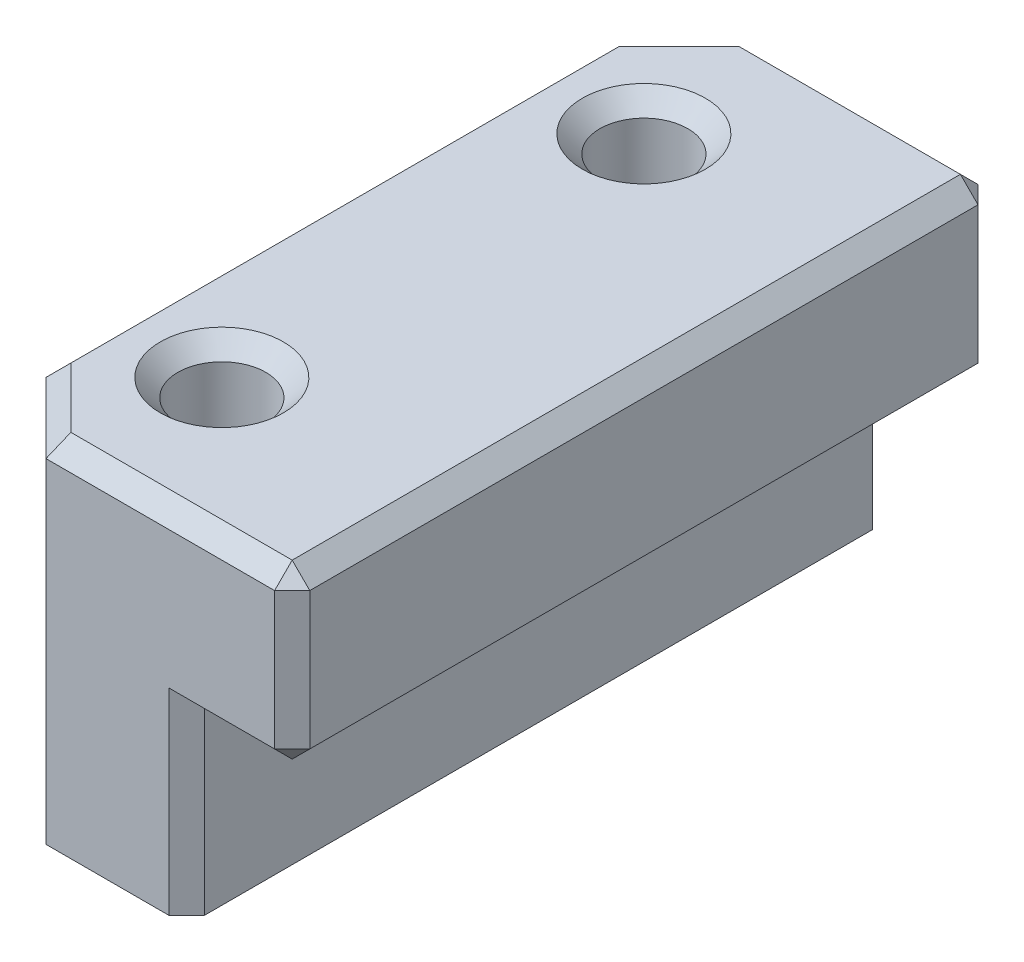
SolidWorks part; units mm, degrees
material "45#"
ref_plane "前视基准面" through (0, 0, 0) normal (0, 0, 1) x (1, 0, 0)
ref_plane "上视基准面" through (0, 0, 0) normal (0, 1, 0) x (1, 0, 0)
ref_plane "右视基准面" through (0, 0, 0) normal (1, 0, 0) x (0, 0, -1)
sketch "草图1" plane through (0, 0, 0) normal (0, 0, 1) x (1, 0, 0)
  line L0 (0, 0) -> (6, 0)
  line L1 (6, 0) -> (6, 5.1)
  line L2 (6, 5.1) -> (9, 5.1)
  line L3 (9, 5.1) -> (9, 10)
  line L4 (9, 10) -> (0, 10)
  line L5 (0, 10) -> (0, 0)
  dimension "D1" = 10
  dimension "D2" = 5.1
  dimension "D3" = 6
  dimension "D4" = 9
extrude "凸台-拉伸1" add sketch "草图1" along normal blind 20
hole_wizard "M3 螺纹孔1" positions "草图3" profile "草图4" tap size "M3" standard "AS" end condition through all
sketch "草图3" plane through (0, 10, 0) normal (0, 1, 0) x (1, 0, 0)
  line L0 (0, -20) -> (0, 0) construction
  line L1 (9, -20) -> (0, -20) construction
  line L2 (9, 0) -> (0, 0) construction
  point P0 (3, -16)
  point P2 (3, -4)
  dimension "D1" = 3
  dimension "D2" = 3
  dimension "D3" = 4
  dimension "D4" = 4
sketch "草图4" plane through (3, 10, 16) normal (1, 0, 0) x (0, 0, 1)
  line L0 (0, 0) -> (0, 10)
  line L1 (0, 10) -> (1.25, 10)
  line L2 (1.25, 10) -> (1.25, 0)
  line L5 (1.25, 0) -> (0, 0)
  line L11 (0, -6.35) -> (0, 107.95) construction
  dimension "通孔螺纹孔钻头直径" = 2.5
  dimension "通孔螺纹孔钻头深度" = 10
cosmetic thread "孔螺蚊线1"
cosmetic thread "孔螺蚊线2"
chamfer "倒角1" distance 2 angle 45 2 edges at (0, 5, 0) (0, 5, 20)
chamfer "倒角2" distance 0.5 angle 45 15 edges at (3, 10, 5.25) (3, 10, 17.25) (9, 10, 10) (5.5, 10, 20) (1, 10, 19) (0, 10, 10) (1, 10, 1) (5.5, 10, 0) (9, 7.55, 20) (9, 7.55, 0) (6, 2.55, 20) (7.5, 5.1, 20) (9, 5.1, 10) (7.5, 5.1, 0) (6, 2.55, 0)
